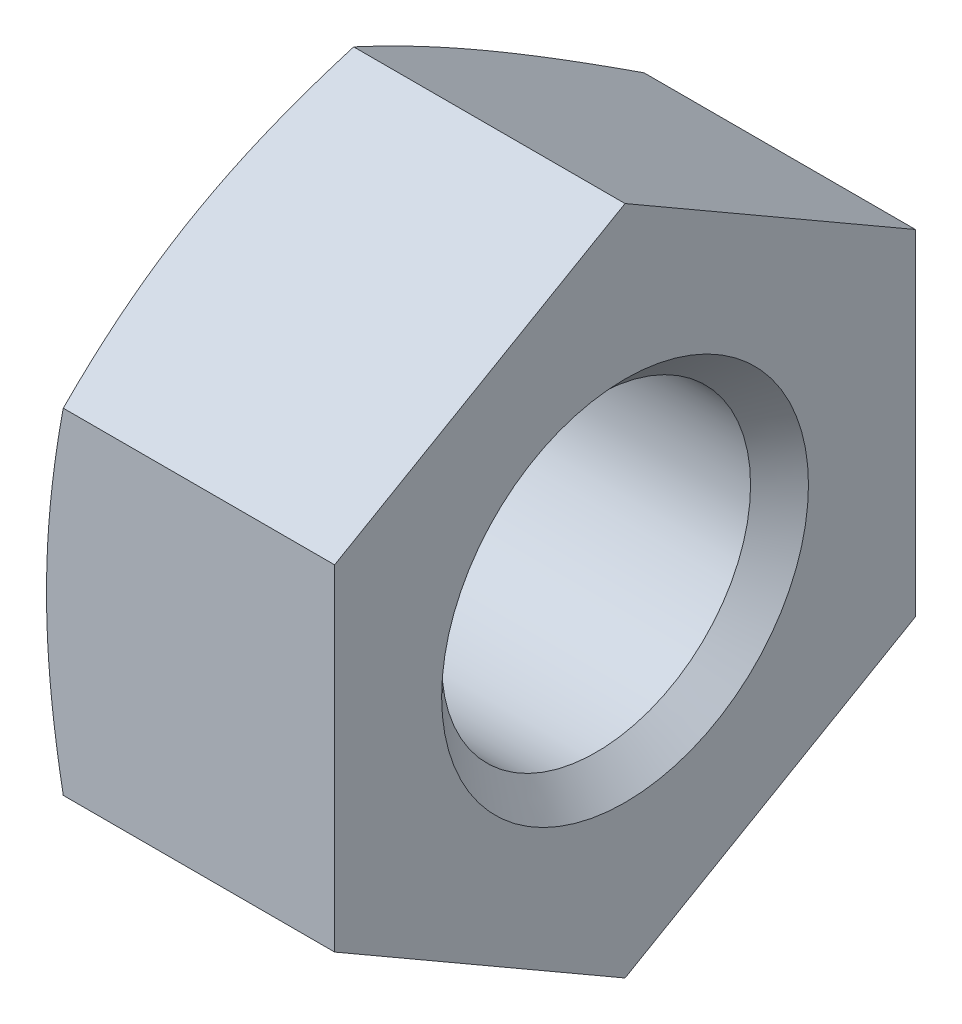
from build123d import *

# Parameters (mm, degrees)
CUT_EXTRUDE_1_DEPTH = 10


with BuildPart() as part:
    # 草图1 → 旋转1 (revolve)
    with BuildSketch(Plane.XY, mode=Mode.PRIVATE) as revolve_1_sk:
        Polygon((0, 7.958333333), (0, 6), (0.947, 5.053), (9.053, 5.053), (10, 6), (10, 11.875), (1.461538462, 11.875), align=None)
    revolve(revolve_1_sk.sketch.rotate(Axis((10, 0, 0), (-1, 0, 0)), 270), axis=Axis((10, 0, 0), (-1, 0, 0)))

    # 草图2 → 切除-拉伸1 (cut)
    with BuildSketch(Plane(origin=(0, 0, 0), x_dir=(0, 0, -1), z_dir=(1, 0, 0))):
        Polygon((-19, 10.969655115), (-19, -10.969655115), (0, -21.939310229), (19, -10.969655115), (19, 10.969655115), (0, 21.939310229), align=None)
        Polygon((-9.5, 5.484827557), (-9.5, -5.484827557), (0, -10.969655115), (9.5, -5.484827557), (9.5, 5.484827557), (0, 10.969655115), align=None, mode=Mode.SUBTRACT)
    extrude(amount=CUT_EXTRUDE_1_DEPTH, mode=Mode.SUBTRACT)


solid = part.part
